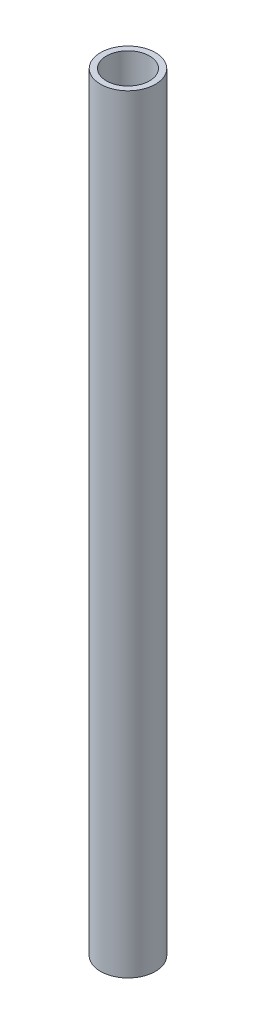
SolidWorks part; units mm, degrees
material "1023 碳钢板 (SS)"
ref_plane "Front Plane" through (0, 0, 0) normal (0, 0, 1) x (1, 0, 0)
ref_plane "Top Plane" through (0, 0, 0) normal (0, 1, 0) x (1, 0, 0)
ref_plane "Right Plane" through (0, 0, 0) normal (1, 0, 0) x (0, 0, -1)
sketch "Sketch1" plane through (0, 0, 0) normal (0, 1, 0) x (1, 0, 0)
  circle A0 centre (0, 0) radius 15
  circle A1 centre (0, 0) radius 11.8
  dimension "D1" = 30
  dimension "D2" = 3.2
extrude "Boss-Extrude1" add sketch "Sketch1" against normal mid plane 420
